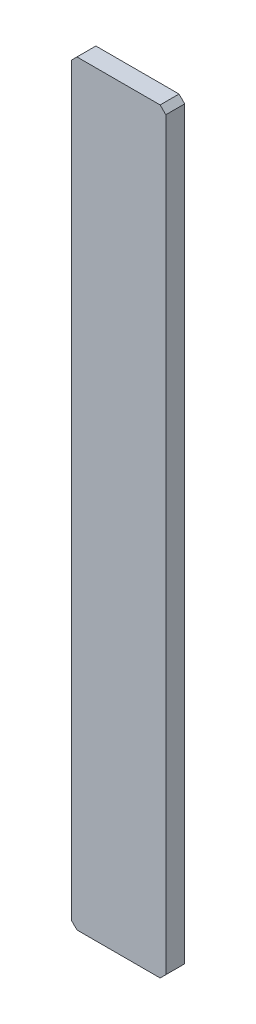
SolidWorks part; units mm, degrees
material "Q235-A"
ref_plane "Front Plane" through (0, 0, 0) normal (0, 0, 1) x (1, 0, 0)
ref_plane "Top Plane" through (0, 0, 0) normal (0, 1, 0) x (1, 0, 0)
ref_plane "Right Plane" through (0, 0, 0) normal (1, 0, 0) x (0, 0, -1)
sketch "Sketch1" plane through (0, 0, 0) normal (0, 0, 1) x (1, 0, 0)
  line L1 (-128.5571, 549.1935) -> (-78.5571, 549.1935)
  line L2 (-128.5571, 549.1935) -> (-128.5571, 149.1935)
  line L3 (-128.5571, 149.1935) -> (-78.5571, 149.1935)
  line L4 (-78.5571, 549.1935) -> (-78.5571, 149.1935)
  dimension "D1" = 50
  dimension "D2" = 400
extrude "Boss-Extrude1" add sketch "Sketch1" along normal blind 10
chamfer "Chamfer1" distance 3 angle 45 4 edges at (-78.5571, 149.1935, 5) (-128.5571, 149.1935, 5) (-128.5571, 549.1935, 5) (-78.5571, 549.1935, 5)
